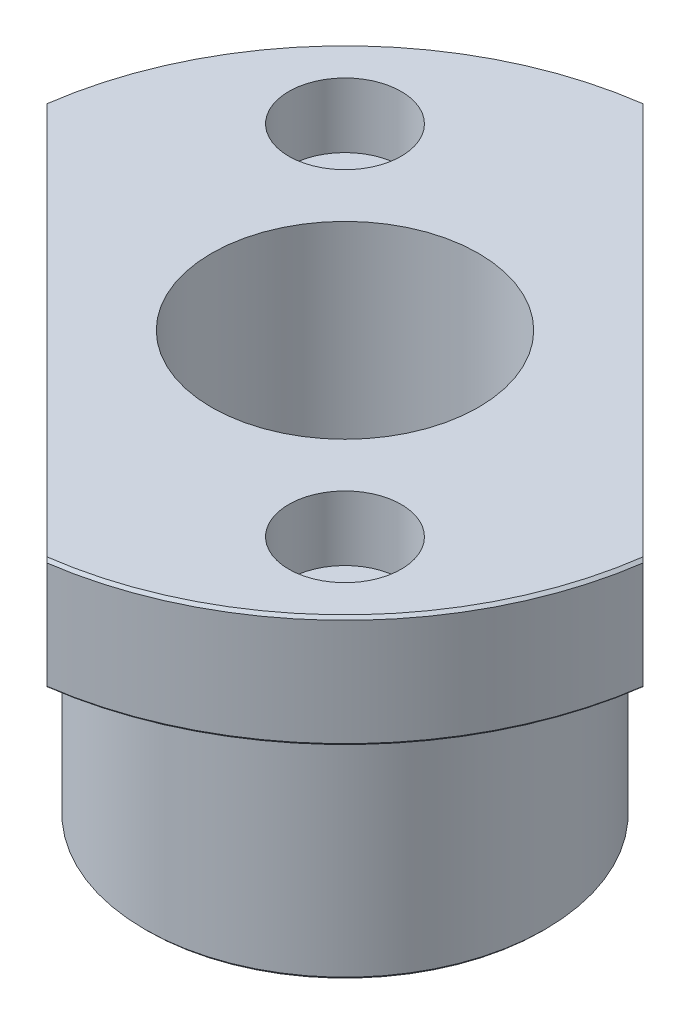
SolidWorks part; units mm, degrees
material "AISI 类型 316L 不锈钢"
ref_plane "Front Plane" through (0, 0, 0) normal (0, 0, 1) x (1, 0, 0)
ref_plane "Top Plane" through (0, 0, 0) normal (0, 1, 0) x (1, 0, 0)
ref_plane "Right Plane" through (0, 0, 0) normal (1, 0, 0) x (0, 0, -1)
sketch "Sketch2" plane through (0, 0, 0) normal (0, 0, 1) x (1, 0, 0)
  line L0 (0, 0) -> (0, 30) construction
  line L1 (0, 30) -> (-25, 30)
  line L2 (-25, 30) -> (-25, 22)
  line L3 (-25, 22) -> (-14.25, 22)
  line L4 (-14.25, 22) -> (-14.25, 0)
  line L5 (-14.25, 0) -> (0, 0)
  line L6 (0, 0) -> (0, 30)
  dimension "D1" = 50
  dimension "D2" = 28.5
  dimension "D3" = 22
  dimension "D4" = 8
revolve "Revolve1" add sketch "Sketch2" angle 360 about L0
hole_wizard "G1/2 Tapped Hole1" positions "3DSketch1" profile "Sketch4" tap size "G1/2" standard "GB" end condition up to next
sketch3d "3DSketch1"
  line L0 (0, 30, 0) -> (0, 22, 0) construction
  point P0 (0, 30, 0)
sketch "Sketch4" plane through (0, 30, 0) normal (1, 0, 0) x (0, 0, 1)
  line L0 (0, 0) -> (0, 30)
  line L1 (0, 30) -> (9.5, 30)
  line L2 (9.5, 30) -> (9.5, 0)
  line L5 (9.5, 0) -> (0, 0)
  line L11 (0, -6.35) -> (0, 107.95) construction
  dimension "通孔螺纹孔钻头直径" = 19
  dimension "通孔螺纹孔钻头深度" = 30
cosmetic thread "Cosmetic Thread 1" parameters "D2"=20.955
sketch "Sketch5" plane through (0, 30, 0) normal (0, 1, 0) x (1, 0, 0)
  line L0 (0, 18) -> (0, -18) construction
  line L1 (18, 0) -> (-18, 0) construction
  line L2 (0, 0) -> (12.7279, 12.7279) construction
  line L3 (0, 0) -> (-12.7279, -12.7279) construction
  line L4 (0, 0) -> (-12.7279, 12.7279) construction
  line L5 (0, 0) -> (12.7279, -12.7279) construction
  circle A0 centre (0, 0) radius 18 construction
  dimension "D1" = 36
  dimension "D2" = 45
  dimension "D3" = 45
hole_wizard "Hole Size (% based on) Socket Head Cap Screw Type 1" positions "3DSketch2" profile "Sketch6" counterbore size "M4" standard "GB" end condition up to next
sketch3d "3DSketch2"
  point P12 (-12.7279, 30, -12.7279)
  point P15 (12.7279, 30, 12.7279)
sketch "Sketch6" plane through (-12.7279, 30, -12.7279) normal (1, 0, 0) x (0, 0, 1)
  line L0 (0, 0) -> (0, 8)
  line L1 (0, 8) -> (2.4, 8)
  line L3 (2.4, 8) -> (2.4, 4.6)
  line L4 (2.4, 4.6) -> (4, 4.6)
  line L5 (4, 4.6) -> (4, 0)
  line L7 (4, 0) -> (0, 0)
  line L11 (0, -6.35) -> (0, 107.95) construction
  dimension "通孔孔直径" = 4.8
  dimension "通孔孔深度" = 8
  dimension "柱形沉头孔直径" = 8
  dimension "柱形沉头孔深度" = 4.6
chamfer "Chamfer1" distance 0.2 angle 45 3 edges at (0, 0, -14.25) (0, 22, -25) (0, 30, -25)
chamfer "Chamfer2" distance 0.2 angle 45 1 edges at (0, 22, -14.25)
sketch "Sketch7" plane through (0, 30, 0) normal (0, 1, 0) x (1, 0, 0)
  line L0 (0, 0) -> (10.6066, 10.6066) construction
  line L1 (0, 0) -> (-10.6066, -10.6066) construction
  line L2 (0, 0) -> (12.7279, -12.7279) construction
  line L3 (-24.7487, 45.9619) -> (45.9619, -24.7487)
  line L4 (24.7487, -45.9619) -> (45.9619, -24.7487)
  line L5 (-45.9619, 24.7487) -> (-24.7487, 45.9619)
  line L6 (0, 0) -> (9, -9) construction
  line L7 (-45.9619, 24.7487) -> (24.7487, -45.9619)
  dimension "D1" = 15
  dimension "D2" = 90
  dimension "D3" = 100
extrude "Cut-Extrude1" cut sketch "Sketch7" against normal blind 50 flip side to cut
